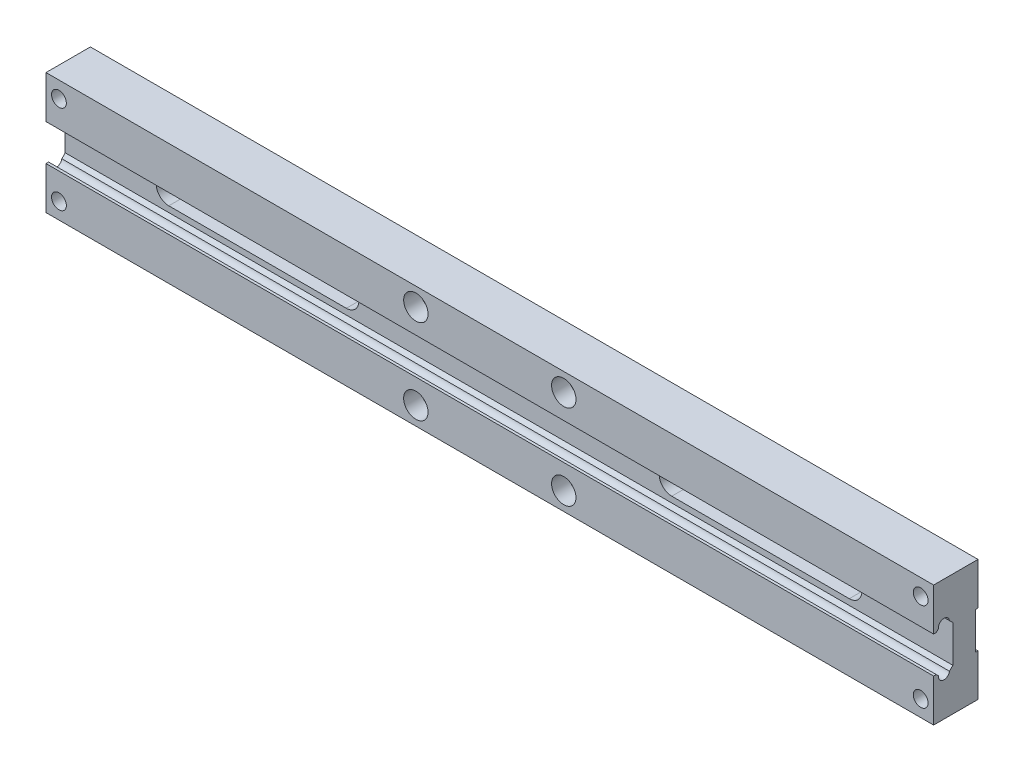
from build123d import *

# Parameters (mm, degrees)
SKETCH_1_W                = 120
SKETCH_1_H                = 16.4
EXTRUDE_1_DEPTH           = 3
SKETCH_2_R                = 1.65
SKETCH_2_R_2              = 1
CUT_EXTRUDE_2_DEPTH       = 2.3
SKETCH_3_R                = 1
CUT_EXTRUDE_3_DEPTH       = 61.854252111
SKETCH_4_W                = 0.35
SKETCH_4_H                = 5
CUT_EXTRUDE_5_DEPTH       = 121.317247309
CUT_EXTRUDE_6_DEPTH       = 61.653112039
CUT_EXTRUDE_7_DEPTH       = 61.854252111
CUT_EXTRUDE_7_DEPTH_BACK  = 61.854252111
SKETCH_7_R                = 1
CUT_EXTRUDE_10_DEPTH      = 61.854252111
CUT_EXTRUDE_10_DEPTH_BACK = 61.854252111
SKETCH_9_R                = 1


with BuildPart() as part:
    # 草图1 → 凸台-拉伸1 (new, symmetric)
    with BuildSketch(Plane.XY):
        Rectangle(SKETCH_1_W, SKETCH_1_H)
    extrude(amount=EXTRUDE_1_DEPTH, both=True)

    # 草图2 → 切除-拉伸2 (cut)
    # profile 1 of 4: a face of its own
    with BuildSketch(Plane.XY.offset(3)):
        with Locations((-10, 5.75)):
            Circle(SKETCH_2_R)
        with Locations((-10, 5.75)):
            Circle(SKETCH_2_R_2, mode=Mode.SUBTRACT)
    # profile 2 of 4: a face of its own
    with BuildSketch(Plane.XY.offset(3)):
        with Locations(Location((10, 5.75, 0), (0, 0, 180))):
            Circle(SKETCH_2_R)
        with Locations(Location((10, 5.75, 0), (0, 0, 180))):
            Circle(SKETCH_2_R_2, mode=Mode.SUBTRACT)
    # profile 3 of 4: a face of its own
    with BuildSketch(Plane.XY.offset(3)):
        with Locations((10, -5.75)):
            Circle(SKETCH_2_R)
        with Locations((10, -5.75)):
            Circle(SKETCH_2_R_2, mode=Mode.SUBTRACT)
    # profile 4 of 4: a face of its own
    with BuildSketch(Plane.XY.offset(3)):
        with Locations(Location((-10, -5.75, 0), (0, 0, 180))):
            Circle(SKETCH_2_R)
        with Locations(Location((-10, -5.75, 0), (0, 0, 180))):
            Circle(SKETCH_2_R_2, mode=Mode.SUBTRACT)
    extrude(amount=-CUT_EXTRUDE_2_DEPTH, mode=Mode.SUBTRACT)

    # 草图3 → 切除-拉伸3 (cut, through all)
    with BuildSketch(Plane.XY.offset(3)):
        with Locations((-10, 5.75)):
            Circle(SKETCH_3_R)
        with Locations((10, 5.75)):
            Circle(SKETCH_3_R)
        with Locations((-10, -5.75)):
            Circle(SKETCH_3_R)
        with Locations((10, -5.75)):
            Circle(SKETCH_3_R)
    extrude(amount=-CUT_EXTRUDE_3_DEPTH, mode=Mode.SUBTRACT)

    # 草图4 → 切除-拉伸5 (cut, through all)
    with BuildSketch(Plane.ZY.offset(60)):
        with Locations((-2.825, 0)):
            Rectangle(SKETCH_4_W, SKETCH_4_H)
        with BuildLine():
            Line((0.4, -2.5), (0.4, 2.5))
            Line((0.4, 2.5), (0.859619408, 2.959619408))
            ThreePointArc((0.859619408, 2.959619408), (1.702223965, 3.593279549), (2.345944084, 2.758335226))
            Line((2.345944084, 2.758335226), (2.65, 2.45427931))
            Line((2.65, 2.45427931), (3, 2.45427931))
            Line((3, 2.45427931), (3, -2.45427931))
            Line((3, -2.45427931), (2.65, -2.45427931))
            Line((2.65, -2.45427931), (2.345944084, -2.758335226))
            ThreePointArc((2.345944084, -2.758335226), (1.702223965, -3.593279549), (0.859619408, -2.959619408))
            Line((0.859619408, -2.959619408), (0.4, -2.5))
        make_face()
    extrude(amount=-CUT_EXTRUDE_5_DEPTH, mode=Mode.SUBTRACT)

    # 草图5 → 切除-拉伸6 (cut, through all)
    with BuildSketch(Plane.XY.offset(0.4)):
        with BuildLine():
            Line((-46, 1.7), (-22, 1.7))
            ThreePointArc((-22, 1.7), (-20.3, 0), (-22, -1.7))
            Line((-22, -1.7), (-46, -1.7))
            ThreePointArc((-46, -1.7), (-47.7, 0), (-46, 1.7))
        make_face()
        with BuildLine():
            Line((46, 1.7), (22, 1.7))
            ThreePointArc((22, 1.7), (20.3, 0), (22, -1.7))
            Line((22, -1.7), (46, -1.7))
            ThreePointArc((46, -1.7), (47.7, 0), (46, 1.7))
        make_face()
    extrude(amount=-CUT_EXTRUDE_6_DEPTH, mode=Mode.SUBTRACT)

    # 草图7 → 切除-拉伸7 (cut, two sides: drawn at the far end of the back side and taken through both)
    with BuildSketch(Plane(origin=(0, 0, -3), x_dir=(-1, 0, 0), z_dir=(0, 0, -1)).offset(-CUT_EXTRUDE_7_DEPTH_BACK)):
        with Locations((-58.249999998, -6)):
            Circle(SKETCH_7_R)
        with Locations((-58.249999998, 6)):
            Circle(SKETCH_7_R)
    extrude(amount=CUT_EXTRUDE_7_DEPTH + CUT_EXTRUDE_7_DEPTH_BACK, mode=Mode.SUBTRACT)

    # 草图9 → 切除-拉伸10 (cut, two sides: drawn at the far end of the back side and taken through both)
    with BuildSketch(Plane.XY.offset(3).offset(-CUT_EXTRUDE_10_DEPTH_BACK)):
        with Locations((-58.249989067, 5.99999379)):
            Circle(SKETCH_9_R)
        with Locations((-58.249989067, -6.00000621)):
            Circle(SKETCH_9_R)
    extrude(amount=CUT_EXTRUDE_10_DEPTH + CUT_EXTRUDE_10_DEPTH_BACK, mode=Mode.SUBTRACT)


solid = part.part
